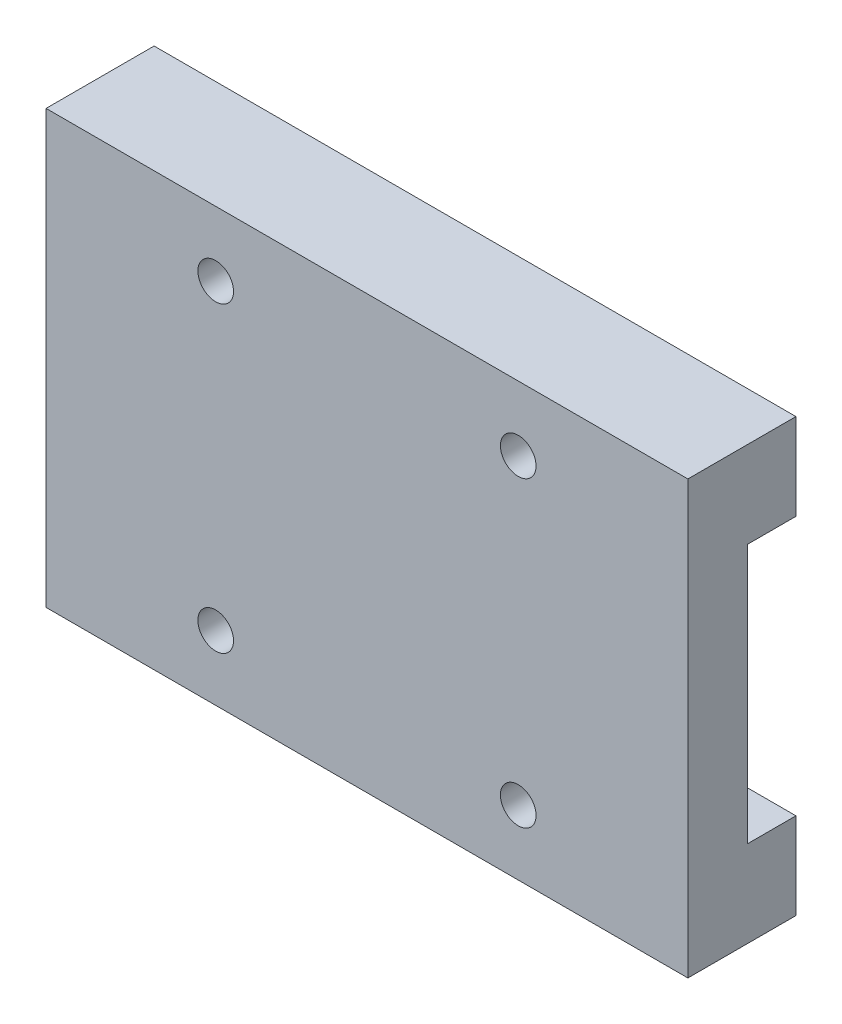
from build123d import *

# Parameters (mm, degrees)
SKETCH1_W             = 59.4
SKETCH1_H             = 40
BOSS_EXTRUDE1_DEPTH   = 10
SKETCH2_W             = 9
SKETCH2_H             = 24
CUT_EXTRUDE1_DEPTH    = 64.469362688
M4_TAPPED_HOLE1_D     = 3.3
M4_TAPPED_HOLE1_DEPTH = 10.1
M4_TAPPED_HOLE1_TIP   = 0.991420021


with BuildPart() as part:
    # Sketch1 → Boss-Extrude1 (new body)
    with BuildSketch(Plane.XY):
        Rectangle(SKETCH1_W, SKETCH1_H)
    extrude(amount=BOSS_EXTRUDE1_DEPTH)

    # Sketch2 → Cut-Extrude1 (cut, through all)
    with BuildSketch(Plane.ZY.offset(29.7)):
        Rectangle(SKETCH2_W, SKETCH2_H)
    extrude(amount=-CUT_EXTRUDE1_DEPTH, mode=Mode.SUBTRACT)

    # M4 Tapped Hole1
    with Locations(Plane.XY.offset(10)):
        with Locations((-14, 14), (14, 14), (14, -14), (-14, -14)):
            Hole(M4_TAPPED_HOLE1_D / 2, depth=M4_TAPPED_HOLE1_DEPTH)
            with Locations((0, 0, -(M4_TAPPED_HOLE1_DEPTH + M4_TAPPED_HOLE1_TIP / 2))):  # 118° drill point
                Cone(0, M4_TAPPED_HOLE1_D / 2, M4_TAPPED_HOLE1_TIP, mode=Mode.SUBTRACT)


solid = part.part
